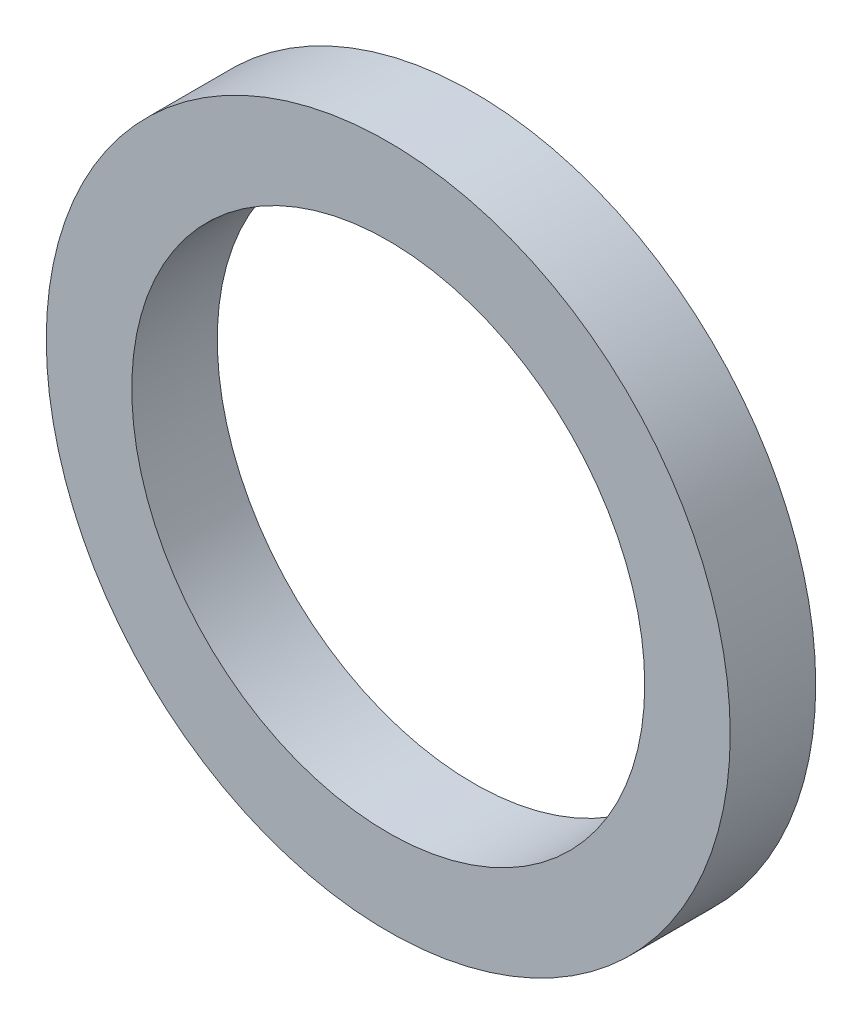
from build123d import *

# Parameters (mm, degrees)
SKETCH1_R           = 4
SKETCH1_R_2         = 3
BOSS_EXTRUDE1_DEPTH = 1


with BuildPart() as part:
    # Sketch1 → Boss-Extrude1 (new body)
    with BuildSketch(Plane.XY):
        Circle(SKETCH1_R)
        Circle(SKETCH1_R_2, mode=Mode.SUBTRACT)
    extrude(amount=BOSS_EXTRUDE1_DEPTH)


solid = part.part
